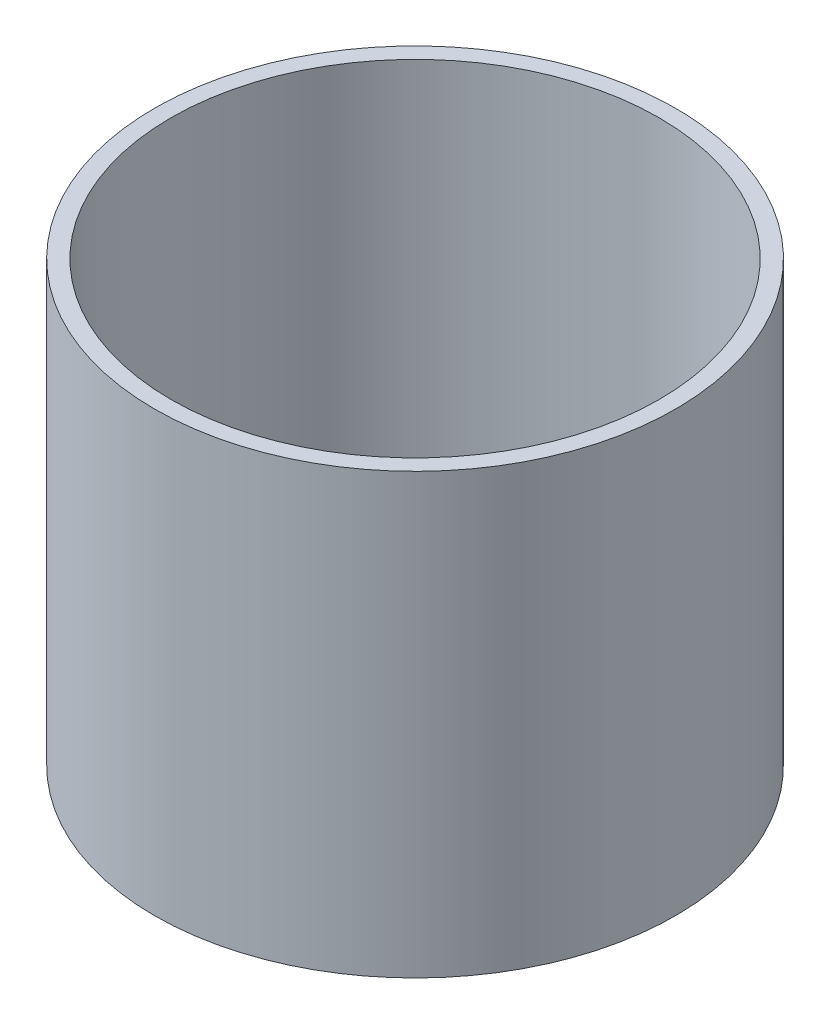
from build123d import *

# Parameters (mm, degrees)
SKETCH_1_R      = 47.5
SKETCH_1_R_2    = 44.5
EXTRUDE_1_DEPTH = 80


with BuildPart() as part:
    # 草图1 → 凸台-拉伸1 (new body)
    with BuildSketch(Plane(origin=(0, 0, 0), x_dir=(1, 0, 0), z_dir=(0, 1, 0))):
        with Locations(Location((0, 0, 0), (0, 0, 270))):
            Circle(SKETCH_1_R)
        with Locations(Location((0, 0, 0), (0, 0, 270))):
            Circle(SKETCH_1_R_2, mode=Mode.SUBTRACT)
    extrude(amount=EXTRUDE_1_DEPTH)


solid = part.part
